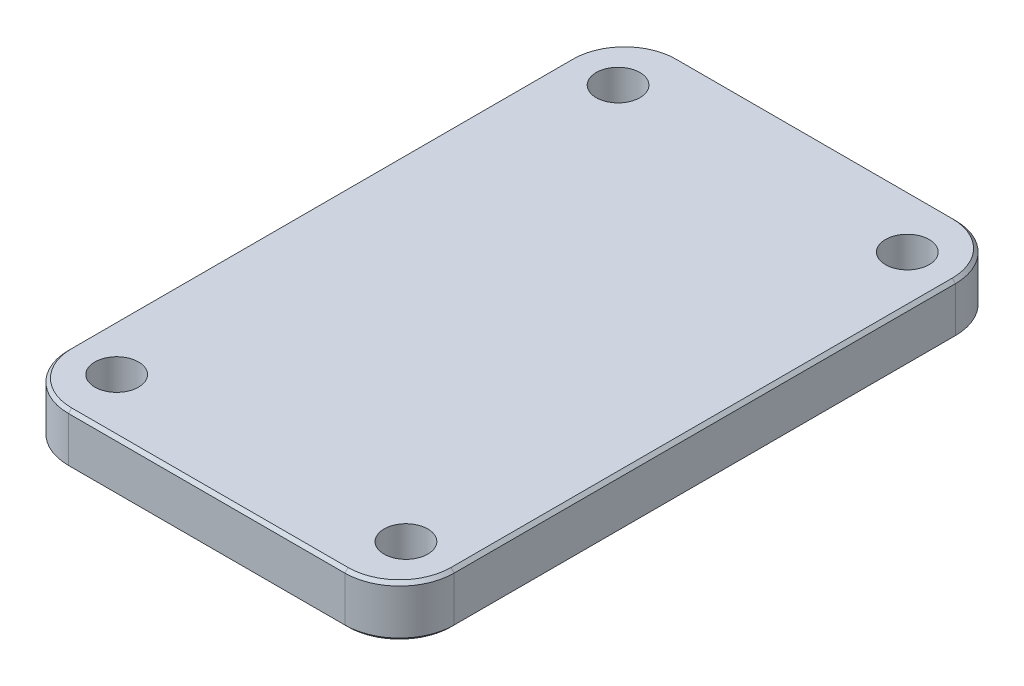
from build123d import *

# Parameters (mm, degrees)
SKETCH1_W                  = 60
SKETCH1_H                  = 95
BOSS_EXTRUDE1_DEPTH        = 8
F_6_8_6_8_DIAMETER_HOLE1_D = 6.8
FILLET1_R                  = 8.5
CHAMFER1_SIZE              = 0.5


with BuildPart() as part:
    # Sketch1 → Boss-Extrude1 (new body)
    with BuildSketch(Plane.XZ.offset(8)):
        with Locations((0, -2.5)):
            Rectangle(SKETCH1_W, SKETCH1_H)
    extrude(amount=-BOSS_EXTRUDE1_DEPTH)

    # Ø6.8 (6.8) Diameter Hole1 (through all)
    with Locations(Plane(origin=(0, -8, 0), x_dir=(-1, 0, 0), z_dir=(0, -1, 0))):
        with Locations((22.5, 41.5), (-22.5, 41.5), (-22.5, -36.5), (22.5, -36.5)):
            Hole(F_6_8_6_8_DIAMETER_HOLE1_D / 2)

    # Fillet1
    fillet1_edges = [part.edges().sort_by_distance(p)[0] for p in [
        (-30, -4, 45),
        (30, -4, 45),
        (30, -4, -50),
        (-30, -4, -50),
    ]]
    fillet(fillet1_edges, radius=FILLET1_R)

    # Chamfer1
    chamfer1_edges = [part.edges().sort_by_distance(p)[0] for p in [
        (0, -8, -50),
        (0, 0, -50),
        (-30, -8, -2.5),
        (30, -8, -2.5),
        (0, -8, 45),
        (-27.51040764, -8, 42.51040764),
        (-27.51040764, -8, -47.51040764),
        (27.51040764, -8, 42.51040764),
        (27.51040764, -8, -47.51040764),
        (30, 0, -2.5),
        (-30, 0, -2.5),
        (0, 0, 45),
        (-27.51040764, 0, 42.51040764),
        (-27.51040764, 0, -47.51040764),
        (27.51040764, 0, 42.51040764),
        (27.51040764, 0, -47.51040764),
    ]]
    chamfer(chamfer1_edges, length=CHAMFER1_SIZE)


solid = part.part
